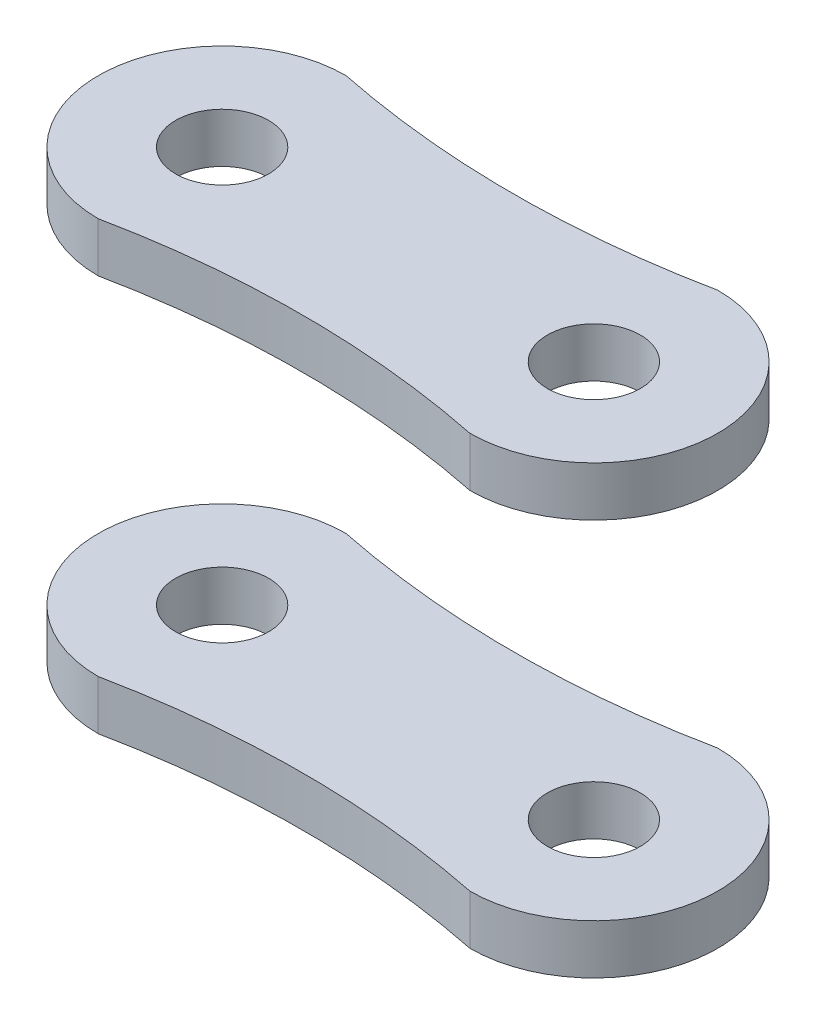
from build123d import *

# Parameters (mm, degrees)
SKETCH1_R           = 7.5
BOSS_EXTRUDE1_DEPTH = 8
LPATTERN1_COUNT     = 2
LPATTERN1_PITCH     = 64


with BuildPart() as part:
    # Sketch1 → Boss-Extrude1 (new body)
    with BuildSketch(Plane(origin=(0, 0, 0), x_dir=(1, 0, 0), z_dir=(0, 1, 0))):
        with BuildLine():
            ThreePointArc((0, 20), (-20, 0), (0, -20))
            ThreePointArc((0, -20), (30, -16.969384567), (60, -20))
            ThreePointArc((60, -20), (80, 0), (60, 20))
            ThreePointArc((60, 20), (30, 16.969384567), (0, 20))
        make_face()
        with Locations(Location((0, 0, 0), (0, 0, 270))):
            Circle(SKETCH1_R, mode=Mode.SUBTRACT)
        with Locations(Location((60, 0, 0), (0, 0, 270))):
            Circle(SKETCH1_R, mode=Mode.SUBTRACT)
    extrude(amount=BOSS_EXTRUDE1_DEPTH)


with BuildPart() as lpattern1_1:
    # LPattern1: pattern copy
    add(part.part.moved(Location(Vector(0, 1, 0) * (1 * LPATTERN1_PITCH))))


solid = Compound([part.part, lpattern1_1.part])
